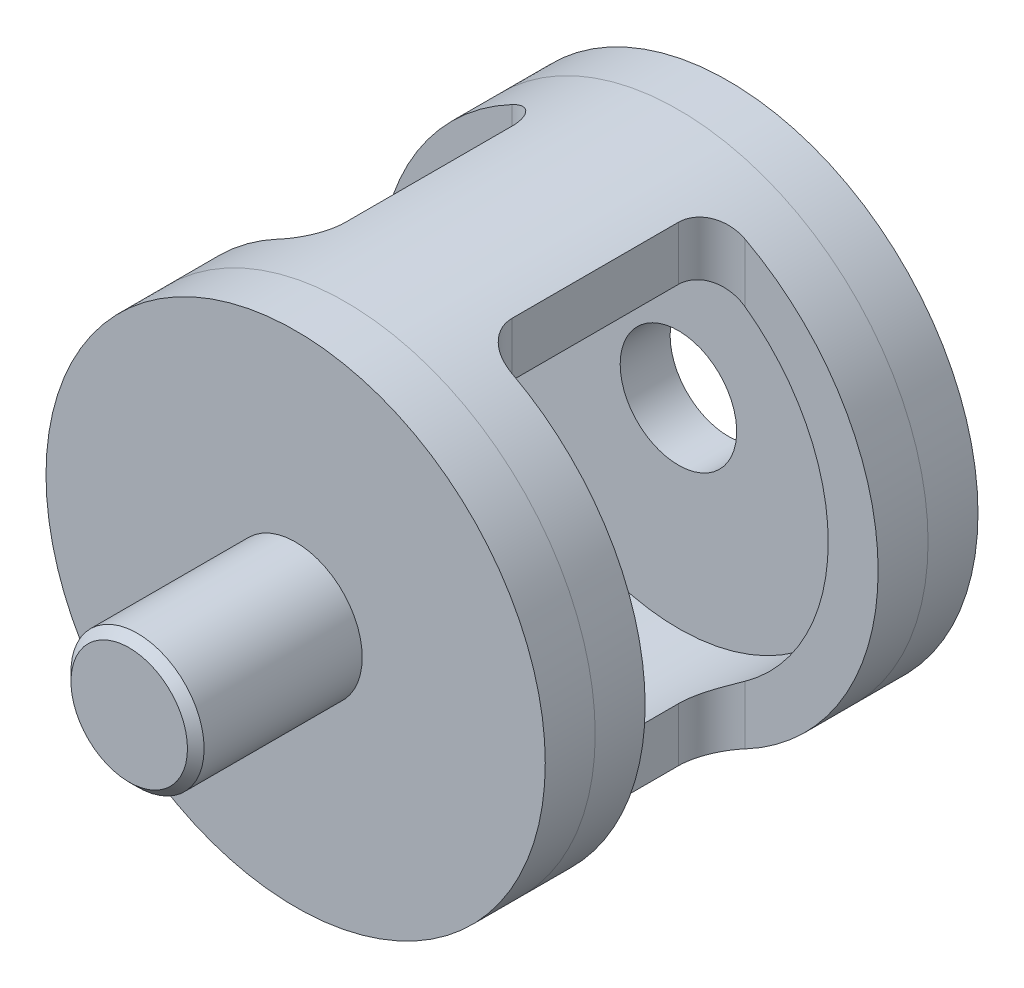
from build123d import *

# Parameters (mm, degrees)
SKETCH1_R               = 15
SKETCH1_R_2             = 12
BOSS_EXTRUDE1_DEPTH     = 20
CUT_EXTRUDE1_DEPTH      = 30.154759474
CUT_EXTRUDE1_DEPTH_BACK = 30.154759474
SKETCH2_W               = 10
SKETCH2_H               = 14
SKETCH3_R               = 15
BOSS_EXTRUDE2_DEPTH     = 3
SKETCH5_R               = 15
BOSS_EXTRUDE3_DEPTH     = 3
SKETCH11_R              = 4
BOSS_EXTRUDE4_DEPTH     = 10
FILLET1_R               = 2
CHAMFER1_SIZE           = 0.5


with BuildPart() as part:
    # Sketch1 → Boss-Extrude1 (new body)
    with BuildSketch(Plane.XY):
        Circle(SKETCH1_R)
        Circle(SKETCH1_R_2, mode=Mode.SUBTRACT)
    extrude(amount=BOSS_EXTRUDE1_DEPTH)

    # Sketch2 → Cut-Extrude1 (cut, two sides: drawn at the far end of the back side and taken through both)
    with BuildSketch(Plane(origin=(0, 0, 0), x_dir=(1, 0, 0), z_dir=(0, 1, 0)).offset(-CUT_EXTRUDE1_DEPTH_BACK)):
        with Locations((-10, -10)):
            Rectangle(SKETCH2_W, SKETCH2_H)
        with Locations((10, -10)):
            Rectangle(SKETCH2_W, SKETCH2_H)
    extrude(amount=CUT_EXTRUDE1_DEPTH + CUT_EXTRUDE1_DEPTH_BACK, mode=Mode.SUBTRACT)

    # Fillet1
    fillet1_edges = [part.edges().sort_by_distance(p)[0] for p in [
        (-5, -12.525423869, 3),
        (-5, 12.525423869, 3),
        (-5, 12.525423869, 17),
        (-5, -12.525423869, 17),
        (5, 12.525423869, 3),
        (5, -12.525423869, 3),
        (5, 12.525423869, 17),
        (5, -12.525423869, 17),
    ]]
    fillet(fillet1_edges, radius=FILLET1_R)


with BuildPart() as body_2:
    # Sketch3 → Boss-Extrude2 (new body)
    with BuildSketch(Plane.XY.offset(20)):
        Circle(SKETCH3_R)
    extrude(amount=BOSS_EXTRUDE2_DEPTH)

    # Sketch10 → M8 Tapped Hole1 (revolve, cut)
    with BuildSketch(Plane(origin=(0, 0, 23), x_dir=(0, -1, 0), z_dir=(1, 0, 0))):
        Polygon((0, 0), (0, 12.042926105), (3.4, 10), (3.4, 0), align=None)
    revolve(axis=Axis((0, 0, 29.35), (0, 0, -1)), mode=Mode.SUBTRACT)

    # Sketch11 → Boss-Extrude4 (add)
    with BuildSketch(Plane.XY.offset(23)):
        Circle(SKETCH11_R)
    extrude(amount=BOSS_EXTRUDE4_DEPTH)

    # Chamfer1
    chamfer1_edges = [body_2.edges().sort_by_distance(p)[0] for p in [
        (-4, 0, 33),
    ]]
    chamfer(chamfer1_edges, length=CHAMFER1_SIZE)


with BuildPart() as body_3:
    # Sketch5 → Boss-Extrude3 (new body)
    with BuildSketch(Plane(origin=(0, 0, 0), x_dir=(-1, 0, 0), z_dir=(0, 0, -1))):
        Circle(SKETCH5_R)
    extrude(amount=BOSS_EXTRUDE3_DEPTH)

    # Sketch8 → M6 Clearance Hole1 (revolve, cut)
    with BuildSketch(Plane(origin=(0, 0, -3), x_dir=(0, 1, 0), z_dir=(1, 0, 0))):
        Polygon((0, 0), (0, 7.103012167), (3.5, 5), (3.5, 0), align=None)
    revolve(axis=Axis((0, 0, -9.35), (0, 0, 1)), mode=Mode.SUBTRACT)


solid = Compound([part.part, body_2.part, body_3.part])
